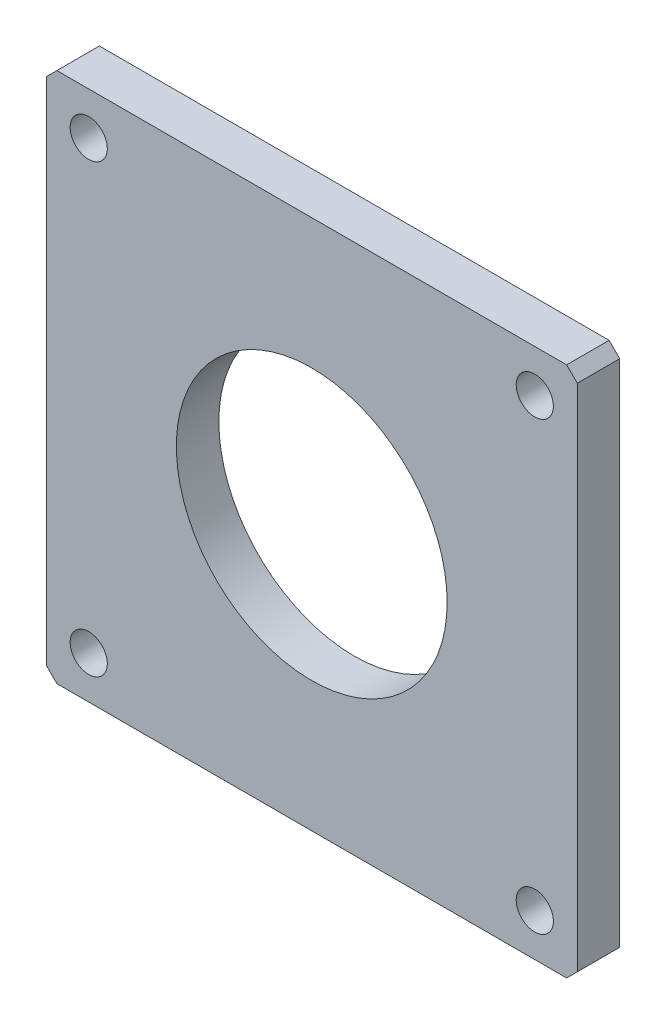
SolidWorks part; units mm, degrees
ref_plane "前视基准面" through (0, 0, 0) normal (0, 0, 1) x (1, 0, 0)
ref_plane "上视基准面" through (0, 0, 0) normal (0, 1, 0) x (1, 0, 0)
ref_plane "右视基准面" through (0, 0, 0) normal (1, 0, 0) x (0, 0, -1)
sketch "草图1" plane through (0, 0, 0) normal (0, 0, 1) x (1, 0, 0)
  line L1 (-50, -50) -> (50, -50)
  line L2 (-50, -50) -> (-50, 50)
  line L3 (-50, 50) -> (50, 50)
  line L4 (50, -50) -> (50, 50)
  line L5 (-50, -50) -> (50, 50) construction
  line L6 (-50, 50) -> (50, -50) construction
  point P0 (0, 0)
  dimension "D1" = 100
extrude "凸台-拉伸1" add sketch "草图1" along normal blind 8
sketch "草图2" plane through (0, 0, 8) normal (0, 0, 1) x (1, 0, 0)
  circle A0 centre (0, 0) radius 25.5
  dimension "D1" = 51
extrude "切除-拉伸1" cut sketch "草图2" against normal up to next
sketch "草图3" plane through (0, 0, 8) normal (0, 0, 1) x (1, 0, 0)
  line L0 (50, 50) -> (-50, 50) construction
  line L1 (-50, 50) -> (-50, -50) construction
  circle A0 centre (-42, 42) radius 3.5
  dimension "D1" = 7
  dimension "D2" = 8
  dimension "D3" = 8
extrude "切除-拉伸2" cut sketch "草图3" against normal up to next
pattern_circular "阵列(圆周)1" count 4 over 360 about axis through (0, 0, 0) along (0, 0, 1) of "切除-拉伸2"
chamfer "倒角1" distance 2 angle 45 4 edges at (50, 50, 4) (-50, 50, 4) (50, -50, 4) (-50, -50, 4)
